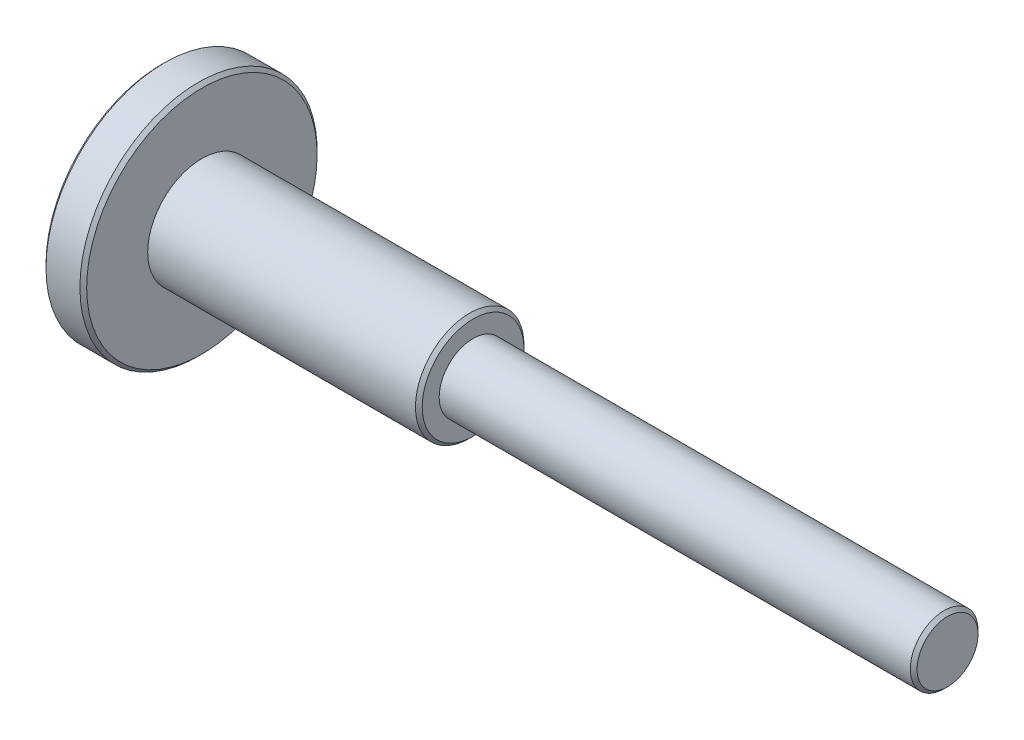
SolidWorks part; units mm, degrees
material "45(Ni)"
ref_plane "Front Plane" through (0, 0, 0) normal (0, 0, 1) x (1, 0, 0)
ref_plane "Top Plane" through (0, 0, 0) normal (0, 1, 0) x (1, 0, 0)
ref_plane "Right Plane" through (0, 0, 0) normal (1, 0, 0) x (0, 0, -1)
sketch "Sketch1" plane through (0, 0, 0) normal (0, 0, 1) x (1, 0, 0)
  line L0 (0, 0) -> (296.6277, 0) construction
  line L1 (0, 0) -> (0, 17.5)
  line L2 (0, 17.5) -> (6, 17.5)
  line L3 (6, 17.5) -> (6, 8)
  line L4 (6, 8) -> (46, 8)
  line L5 (46, 8) -> (46, 5)
  line L6 (46, 5) -> (116, 5)
  line L7 (116, 5) -> (116, 0)
  line L8 (116, 0) -> (0, 0)
  dimension "D1" = 35
  dimension "D2" = 16
  dimension "D3" = 10
  dimension "D4" = 6
  dimension "D5" = 40
  dimension "D6" = 70
revolve "Revolve1" add sketch "Sketch1" angle 360 about L0
cosmetic thread "Cosmetic Thread1" parameters "D1"=20, "D2"=9
chamfer "Chamfer1" distance 0.5 angle 45 3 edges at (46, 0, 8) (6, 0, 17.5) (0, 0, 17.5)
chamfer "Chamfer2" distance 0.5 angle 45 1 edges at (116, 0, 5)
